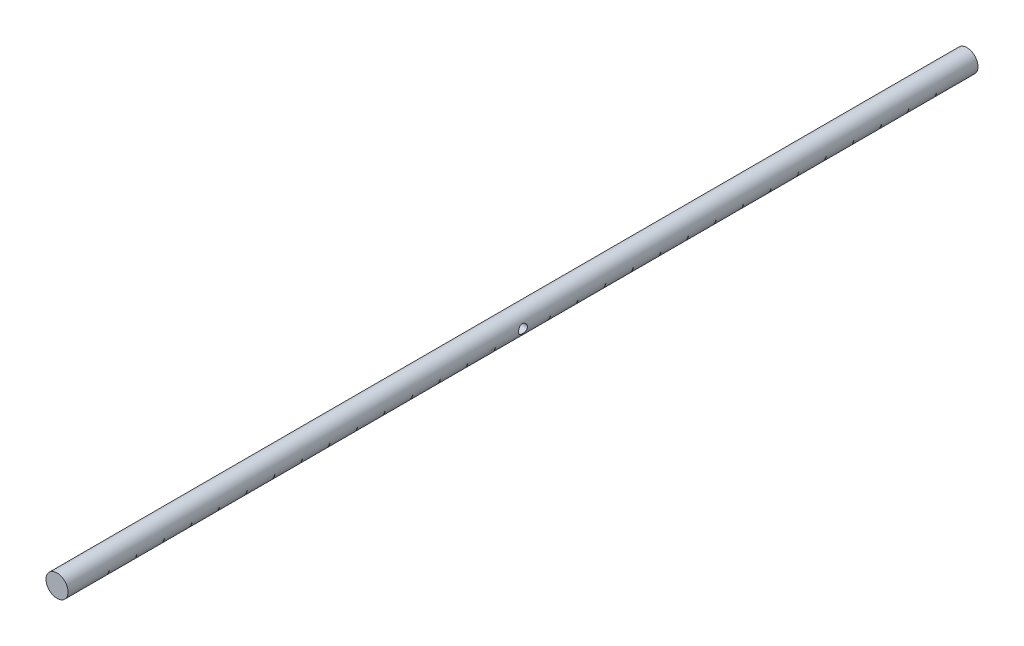
SolidWorks part; units mm, degrees
ref_plane "Front Plane" through (0, 0, 0) normal (0, 0, 1) x (1, 0, 0)
ref_plane "Top Plane" through (0, 0, 0) normal (0, 1, 0) x (1, 0, 0)
ref_plane "Right Plane" through (0, 0, 0) normal (1, 0, 0) x (0, 0, -1)
sketch "Sketch1" plane through (0, 0, 0) normal (0, 0, 1) x (1, 0, 0)
  circle A0 centre (0, 0) radius 4
extrude "Boss-Extrude1" add sketch "Sketch1" along normal blind 330
ref_plane "Plane1" through (4, 0, 0) normal (1, 0, 0) x (0, 0, -1)
sketch "Sketch2" plane through (4, 0, 0) normal (1, 0, 0) x (0, 0, -1)
  line L0 (0, 0) -> (-330, 0) construction
  line L1 (-330, 4) -> (-330, -4) construction
  circle A0 centre (-165, 0) radius 1.6
  dimension "D1" = 3.2
extrude "Cut-Extrude1" cut sketch "Sketch2" against normal through all
ref_plane "Plane2" through (0, 0, 165) normal (0, 0, 1) x (1, 0, 0)
sketch "Sketch6" plane through (0, 0, 165) normal (0, 0, -1) x (-1, 0, 0)
  line L0 (0, 0) -> (-5.3659, 0) construction
  line L1 (0, 0) -> (0, -5.1008) construction
  line L2 (0, -3.9) -> (0, -4.5) construction
  line L3 (-2.9876, -2.5069) -> (-3.4472, -2.8925)
  line L4 (0, -3.9) -> (0, -4.5)
  line L6 (-2.9876, -2.5069) -> (0, 0) construction
  line L7 (0, -3.9) -> (0, 0) construction
  arc A0 (-3.4472, -2.8925) -> (0, -4.5) centre (0, 0) ccw
  arc A1 (-2.9876, -2.5069) -> (0, -3.9) centre (0, 0) ccw
  dimension "D1" = 9
  dimension "D2" = 7.8
  dimension "D3" = 0
  dimension "D4" = 50
extrude "Cut-Extrude2" cut sketch "Sketch6" against normal mid plane 0.2
pattern_linear "LPattern1" count 31 spacing 5 along (0, 0, -1) count 31 spacing 5 along (0, 0, 1) seed only of "Cut-Extrude2"
sketch "Sketch7" plane through (0, 0, 165) normal (0, 0, 1) x (1, 0, 0)
  line L0 (0, 0) -> (0, -4.7644) construction
  line L1 (0, 0) -> (5.2219, 0) construction
  line L2 (3.4472, -2.8925) -> (2.9876, -2.5069)
  line L3 (0, -3.9) -> (0, -4.5)
  line L6 (-4, 0) -> (4, 0) construction
  line L7 (3.8408, -0.6772) -> (4.4316, -0.7814)
  line L9 (0, 0) -> (5.7045, -1.0059) construction
  line L10 (0, -4.5) -> (0, -3.9)
  line L12 (0, -3.9) -> (0, -4.5) construction
  arc A2 (0, -4.5) -> (3.4472, -2.8925) centre (0, 0) ccw
  arc A3 (0, -3.9) -> (2.9876, -2.5069) centre (0, 0) ccw
  arc A4 (0, -4.5) -> (4.4316, -0.7814) centre (0, 0) ccw
  arc A5 (0, -3.9) -> (3.8408, -0.6772) centre (0, 0) ccw
  dimension "D2" = 80
  dimension "D1" = 0
extrude "Cut-Extrude3" cut sketch "Sketch7" against normal mid plane 0.2
pattern_linear "LPattern2" count 16 spacing 10 along (0, 0, 1) count 16 spacing 10 along (0, 0, -1) seed only of "Cut-Extrude3"
